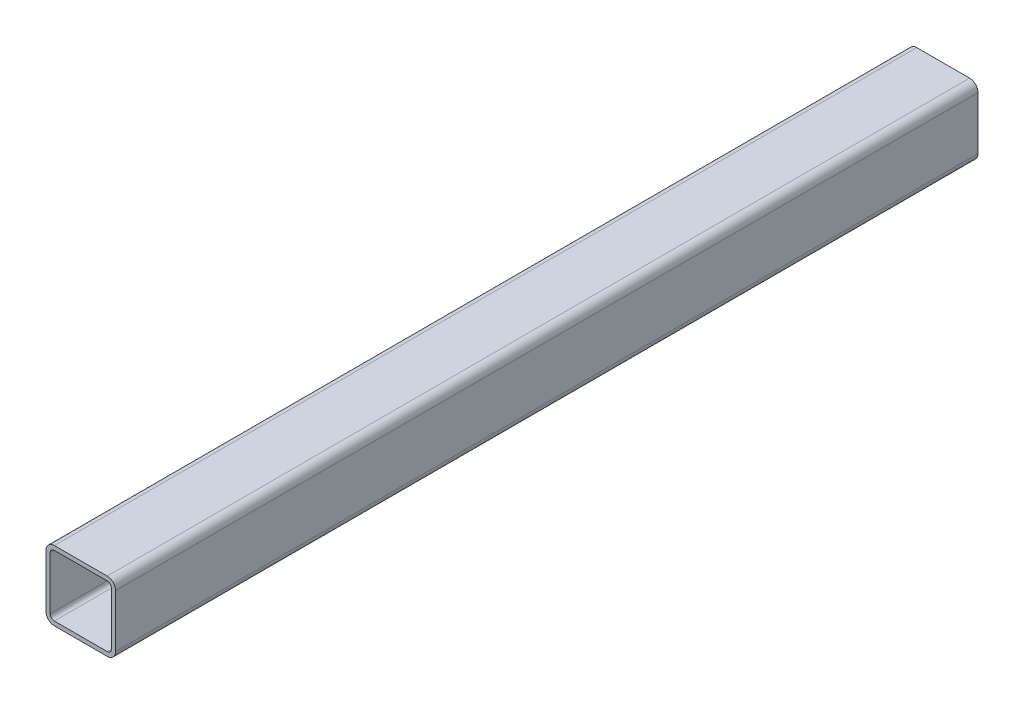
from build123d import *

# Parameters (mm, degrees)
GB_6728_1986_050_X_50_X_3_1_DEPTH = 620


with BuildPart() as part:
    # Sketch1 → Gb／6728-1986方形空心型钢 050 X 50 X 3(1) (new body)
    with BuildSketch(Plane.YX.offset(-310)):
        with BuildLine():
            Line((-19, -25), (19, -25))
            ThreePointArc((19, -25), (23.242640687, -23.242640687), (25, -19))
            Line((25, -19), (25, 19))
            ThreePointArc((25, 19), (23.242640687, 23.242640687), (19, 25))
            Line((19, 25), (-19, 25))
            ThreePointArc((-19, 25), (-23.242640687, 23.242640687), (-25, 19))
            Line((-25, 19), (-25, -19))
            ThreePointArc((-25, -19), (-23.242640687, -23.242640687), (-19, -25))
        make_face()
        with BuildLine():
            Line((-19, -22), (19, -22))
            ThreePointArc((19, -22), (21.121320344, -21.121320344), (22, -19))
            Line((22, -19), (22, 19))
            ThreePointArc((22, 19), (21.121320344, 21.121320344), (19, 22))
            Line((19, 22), (-19, 22))
            ThreePointArc((-19, 22), (-21.121320344, 21.121320344), (-22, 19))
            Line((-22, 19), (-22, -19))
            ThreePointArc((-22, -19), (-21.121320344, -21.121320344), (-19, -22))
        make_face(mode=Mode.SUBTRACT)
    extrude(amount=GB_6728_1986_050_X_50_X_3_1_DEPTH)


solid = part.part
